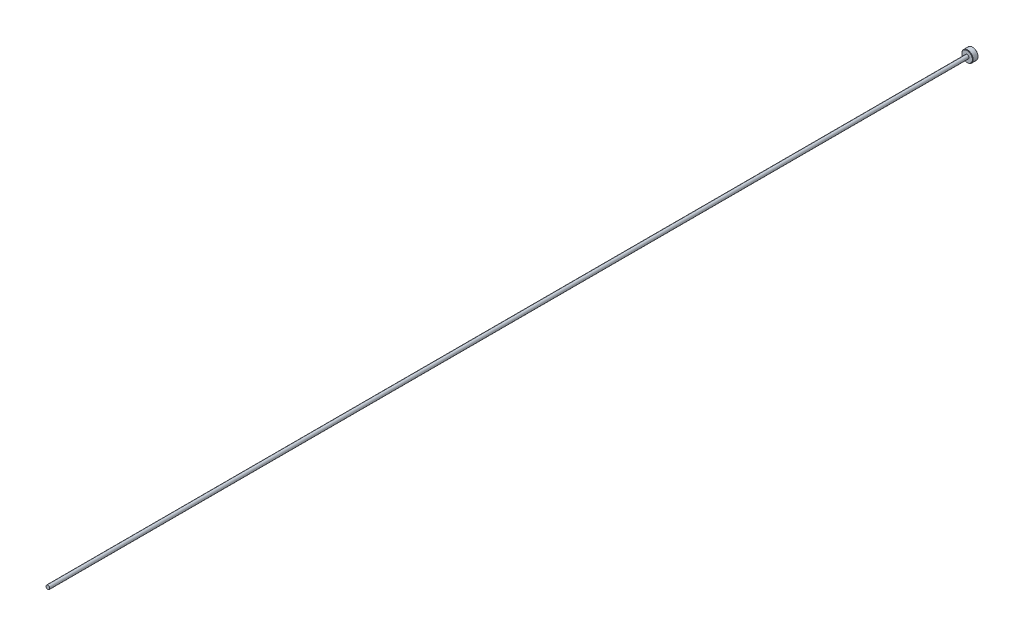
from build123d import *

# Parameters (mm, degrees)
SKETCH1_R           = 1
BOSS_EXTRUDE1_DEPTH = 490
SKETCH2_R           = 3
BOSS_EXTRUDE2_DEPTH = 3
CHAMFER1_SIZE       = 0.2


with BuildPart() as part:
    # Sketch1 → Boss-Extrude1 (new body)
    with BuildSketch(Plane.XY):
        Circle(SKETCH1_R)
    extrude(amount=BOSS_EXTRUDE1_DEPTH)

    # Sketch2 → Boss-Extrude2 (add)
    with BuildSketch(Plane(origin=(0, 0, 0), x_dir=(-1, 0, 0), z_dir=(0, 0, -1))):
        Circle(SKETCH2_R)
    extrude(amount=BOSS_EXTRUDE2_DEPTH)

    # Chamfer1
    chamfer1_edges = [part.edges().sort_by_distance(p)[0] for p in [
        (3, 0, 0),
        (3, 0, -3),
    ]]
    chamfer(chamfer1_edges, length=CHAMFER1_SIZE)


solid = part.part
